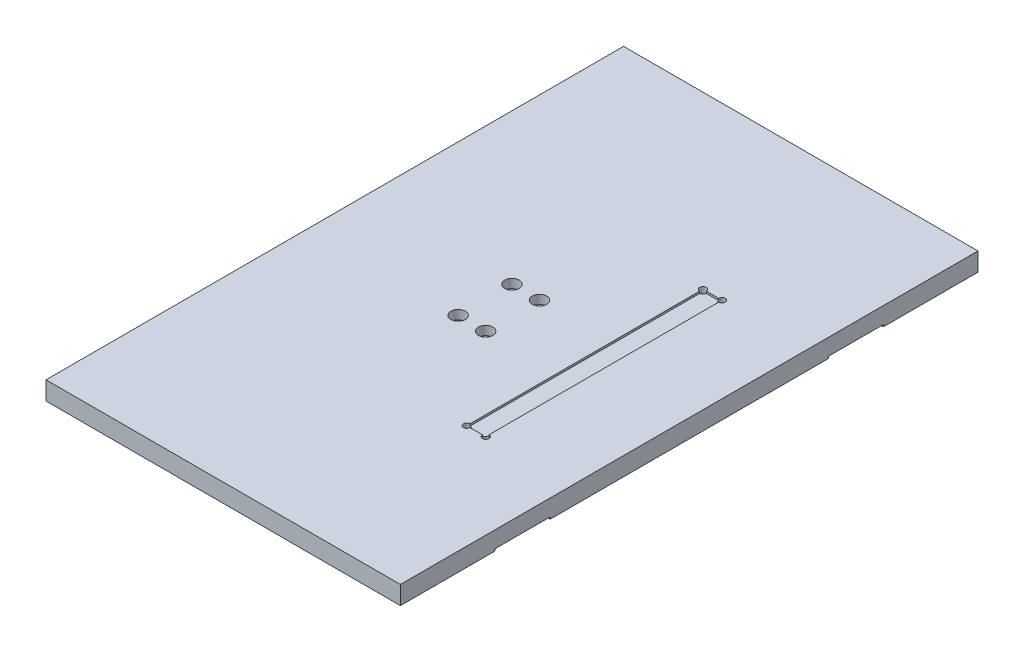
SolidWorks part; units mm, degrees
material "6061 铝合金"
ref_plane "前视基准面" through (0, 0, 0) normal (0, 0, 1) x (1, 0, 0)
ref_plane "上视基准面" through (0, 0, 0) normal (0, 1, 0) x (1, 0, 0)
ref_plane "右视基准面" through (0, 0, 0) normal (1, 0, 0) x (0, 0, -1)
sketch "草图1" plane through (0, 0, 0) normal (0, 1, 0) x (1, 0, 0)
  line L1 (-135, -220) -> (135, -220)
  line L2 (-135, -220) -> (-135, 220)
  line L3 (-135, 220) -> (135, 220)
  line L4 (135, -220) -> (135, 220)
  line L5 (-135, -220) -> (135, 220) construction
  line L6 (-135, 220) -> (135, -220) construction
  point P0 (0, 0)
  dimension "D1" = 440
  dimension "D2" = 270
extrude "凸台-拉伸1" add sketch "草图1" along normal blind 14
sketch "草图2" plane through (0, 0, 0) normal (0, -1, 0) x (1, 0, 0)
  line L0 (135, 220) -> (135, -220) construction
  line L1 (-135, 148) -> (135, 148)
  line L2 (-135, 148) -> (-135, 106)
  line L3 (-135, 106) -> (135, 106)
  line L4 (135, 148) -> (135, 106)
  line L5 (-135, -220) -> (-135, 220) construction
  line L6 (-135, -148) -> (135, -148)
  line L7 (-135, -148) -> (-135, -106)
  line L8 (-135, -106) -> (135, -106)
  line L9 (135, -148) -> (135, -106)
  line L10 (-135, 220) -> (135, 220) construction
  line L11 (135, -220) -> (-135, -220) construction
extrude "切除-拉伸1" cut sketch "草图2" against normal blind 1.5
hole_wizard "打孔尺寸(%根据)内六角圆柱头螺钉的类型1" positions "3D草图1" profile "草图3" counterbore size "M6" standard "GB"
sketch3d "3D草图1"
  circle A0 centre (-20.55, 0, 20.5) radius 3.025 construction
  circle A1 centre (-20.55, -0.525, -20.5) radius 2.5 construction
  circle A2 centre (0.45, 0, 20.5) radius 3.025 construction
  circle A3 centre (0.45, 0, -20.5) radius 3.025 construction
  point P0 (-20.55, 14, 20.5)
  point P2 (-20.55, 14, -20.5)
  point P4 (0.45, 14, 20.5)
  point P6 (0.45, 14, -20.5)
  point P11 (-20.55, 3.025, 20.5)
  point P16 (-20.55, 1.975, -20.5)
  point P20 (0.45, 3.025, 20.5)
  point P24 (0.45, 3.025, -20.5)
sketch "草图3" plane through (-20.55, 14, 20.5) normal (1, 0, 0) x (0, 0, 1)
  line L0 (0, 0) -> (0, 14)
  line L1 (0, 14) -> (3.3, 14)
  line L3 (3.3, 14) -> (3.3, 6.8)
  line L4 (3.3, 6.8) -> (5.5, 6.8)
  line L5 (5.5, 6.8) -> (5.5, 0)
  line L7 (5.5, 0) -> (0, 0)
  line L11 (0, -6.35) -> (0, 107.95) construction
  dimension "通孔孔直径" = 6.6
  dimension "通孔孔深度" = 14
  dimension "柱形沉头孔直径" = 11
  dimension "柱形沉头孔深度" = 6.8
sketch "草图4" plane through (0, 14, 0) normal (0, 1, 0) x (1, 0, 0)
  line L1 (70, -90) -> (55.5, -90)
  line L2 (70, -90) -> (70, 90)
  line L3 (70, 90) -> (55.5, 90)
  line L4 (55.5, -90) -> (55.5, 90)
  line L6 (135, -220) -> (135, 220) construction
  line L7 (-135, 0) -> (55.5, 0) construction
  line L8 (-135, 220) -> (-135, -220) construction
  dimension "D1" = 14.5
  dimension "D2" = 65
  dimension "D3" = 180
extrude "切除-拉伸2" cut sketch "草图4" against normal blind 1.5
sketch "草图5" plane through (0, 14, 0) normal (0, 1, 0) x (1, 0, 0)
  circle A0 centre (55.5, 90) radius 2.5
  circle A1 centre (70, 90) radius 2.5
  circle A2 centre (55.5, -90) radius 2.5
  circle A3 centre (70, -90) radius 2.5
  dimension "D1" = 5
extrude "切除-拉伸3" cut sketch "草图5" against normal up to next
equation "\"D3@草图2\"=\"D2@草图2\""
